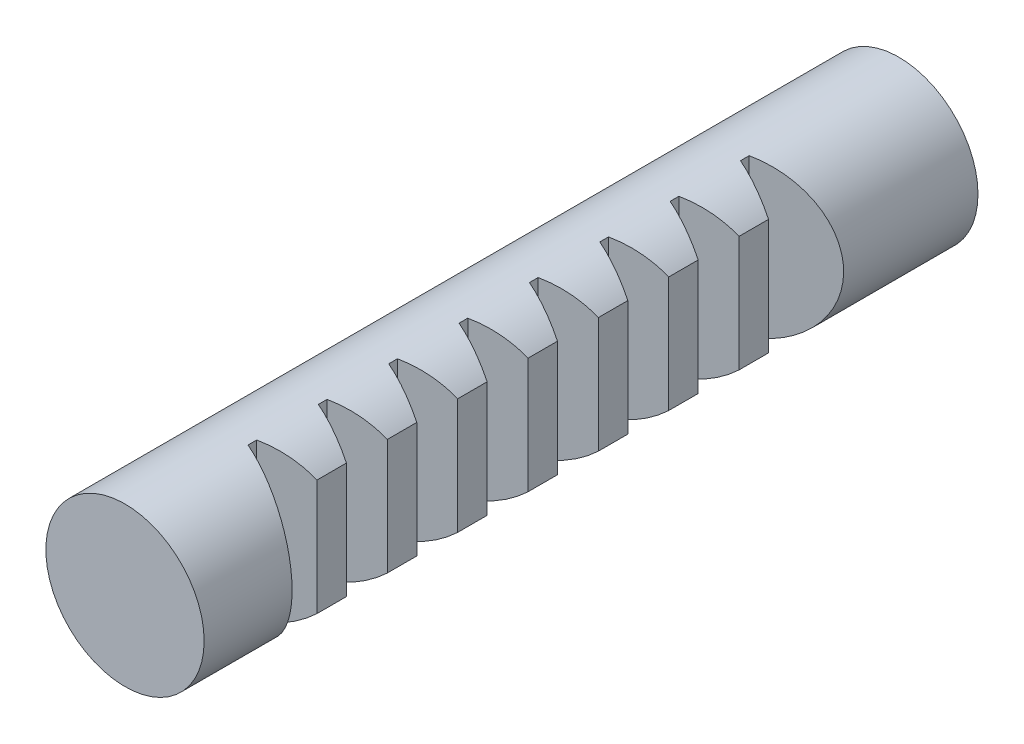
from build123d import *

# Parameters (mm, degrees)
SKETCH1_R               = 9
BOSS_EXTRUDE1_DEPTH     = 44
CUT_EXTRUDE1_DEPTH      = 46.803929962
LPATTERN1_COUNT         = 8
LPATTERN1_PITCH         = 8
CUT_EXTRUDE2_DEPTH      = 46.803929962
CUT_EXTRUDE2_DEPTH_BACK = 46.803929962
SKETCH4_W               = 11.104020724
SKETCH4_H               = 55.76293723


with BuildPart() as part:
    # Sketch1 → Boss-Extrude1 (new, symmetric)
    with BuildSketch(Plane.XY):
        Circle(SKETCH1_R)
    extrude(amount=BOSS_EXTRUDE1_DEPTH, both=True)

    # Sketch2 → Cut-Extrude1 (cut, symmetric)
    with BuildSketch(Plane(origin=(0, 0, 0), x_dir=(1, 0, 0), z_dir=(0, 1, 0))):
        Polygon((9, -34), (1.125, -31.133734405), (1.125, -30.143622784), (9, -27.277357189), align=None)
    cut_extrude1 = extrude(amount=CUT_EXTRUDE1_DEPTH, both=True, mode=Mode.SUBTRACT)

    # LPattern1: Cut-Extrude1 ×8
    with Locations(*[(0, 0, -i * LPATTERN1_PITCH) for i in range(1, LPATTERN1_COUNT)]):
        add(cut_extrude1, mode=Mode.SUBTRACT)

    # Sketch4 → Cut-Extrude2 (cut, two sides: drawn at the far end of the back side and taken through both)
    with BuildSketch(Plane(origin=(0, 0, 0), x_dir=(1, 0, 0), z_dir=(0, 1, 0)).offset(-CUT_EXTRUDE2_DEPTH_BACK)):
        with Locations((11.693935952, -1.197060718)):
            Rectangle(SKETCH4_W, SKETCH4_H)
    extrude(amount=CUT_EXTRUDE2_DEPTH + CUT_EXTRUDE2_DEPTH_BACK, mode=Mode.SUBTRACT)


solid = part.part
